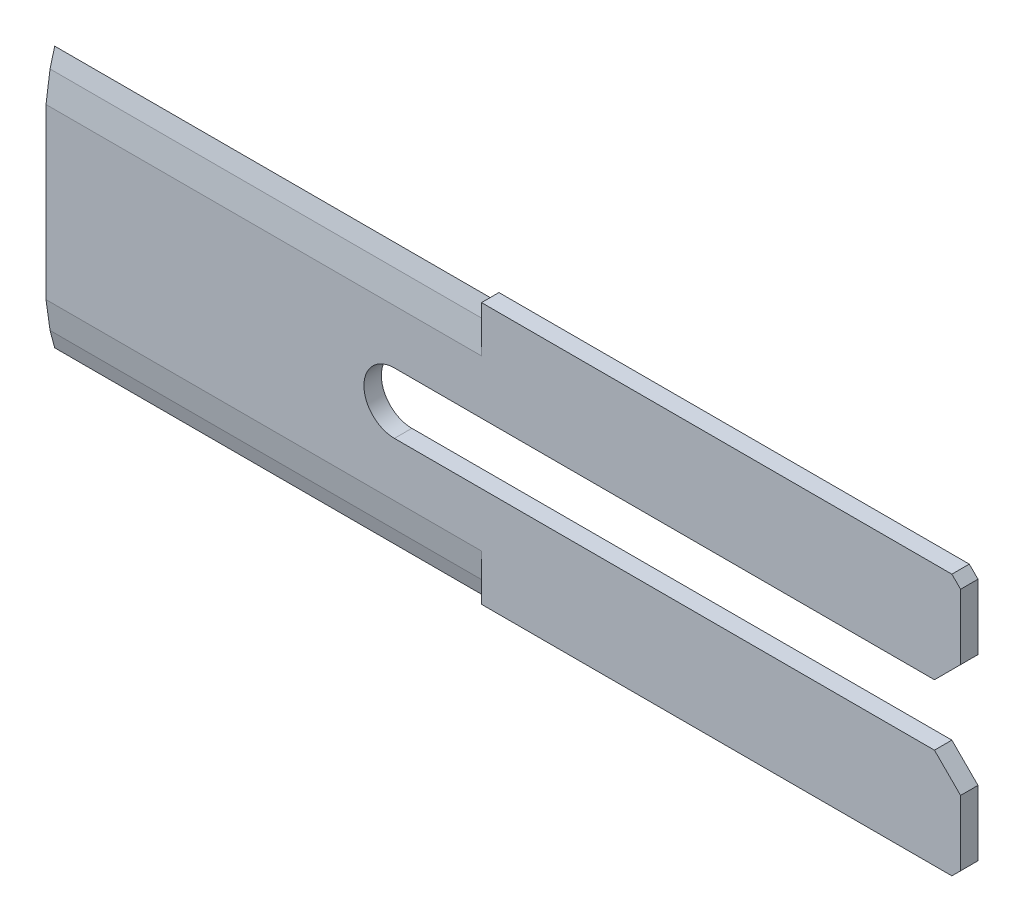
from build123d import *

# Parameters (mm, degrees)
SKETCH_2_W               = 105
SKETCH_2_H               = 30
EXTRUDE_1_DEPTH          = 2
CUT_EXTRUDE_1_DEPTH      = 55.637441375
CUT_EXTRUDE_1_DEPTH_BACK = 55.637441375
SKETCH_5_OUTSIDE_W       = 25.844
SKETCH_5_OUTSIDE_H       = 53.844
CUT_EXTRUDE_7_DEPTH      = 50
CHAMFER_1_SIZE           = 1
CHAMFER_2_SIZE           = 3


with BuildPart() as part:
    # 草图2 → 凸台-拉伸1 (new body)
    with BuildSketch(Plane.XY):
        Rectangle(SKETCH_2_W, SKETCH_2_H)
    extrude(amount=EXTRUDE_1_DEPTH)

    # 草图3 → 切除-拉伸1 (cut, two sides: drawn at the far end of the back side and taken through both)
    with BuildSketch(Plane.XY.offset(2).offset(-CUT_EXTRUDE_1_DEPTH_BACK)):
        with BuildLine():
            Line((52.5, 3.5), (-12.5, 3.5))
            ThreePointArc((-12.5, 3.5), (-16, 0), (-12.5, -3.5))
            Line((-12.5, -3.5), (52.5, -3.5))
            Line((52.5, -3.5), (52.5, 3.5))
        make_face()
    extrude(amount=CUT_EXTRUDE_1_DEPTH + CUT_EXTRUDE_1_DEPTH_BACK, mode=Mode.SUBTRACT)

    # 草图5 outside → 切除-拉伸7 (cut)
    with BuildSketch(Plane.ZY.offset(52.5)):
        with Locations((1, 0)):
            Rectangle(SKETCH_5_OUTSIDE_W, SKETCH_5_OUTSIDE_H)
        Polygon((1, 15), (0.464101615, 13), (0, 9.69774542), (0, -9.69774542), (0.464101615, -13), (1, -15), (1.535898385, -13), (2, -9.69774542), (2, 9.69774542), (1.535898385, 13), align=None, mode=Mode.SUBTRACT)
    extrude(amount=-CUT_EXTRUDE_7_DEPTH, mode=Mode.SUBTRACT)

    # 倒角1
    chamfer_1_edges = [part.edges().sort_by_distance(p)[0] for p in [
        (52.5, -15, 1),
        (52.5, 15, 1),
    ]]
    chamfer(chamfer_1_edges, length=CHAMFER_1_SIZE)

    # 倒角2
    chamfer_2_edges = [part.edges().sort_by_distance(p)[0] for p in [
        (52.5, -3.5, 1),
        (52.5, 3.5, 1),
    ]]
    chamfer(chamfer_2_edges, length=CHAMFER_2_SIZE)


solid = part.part
